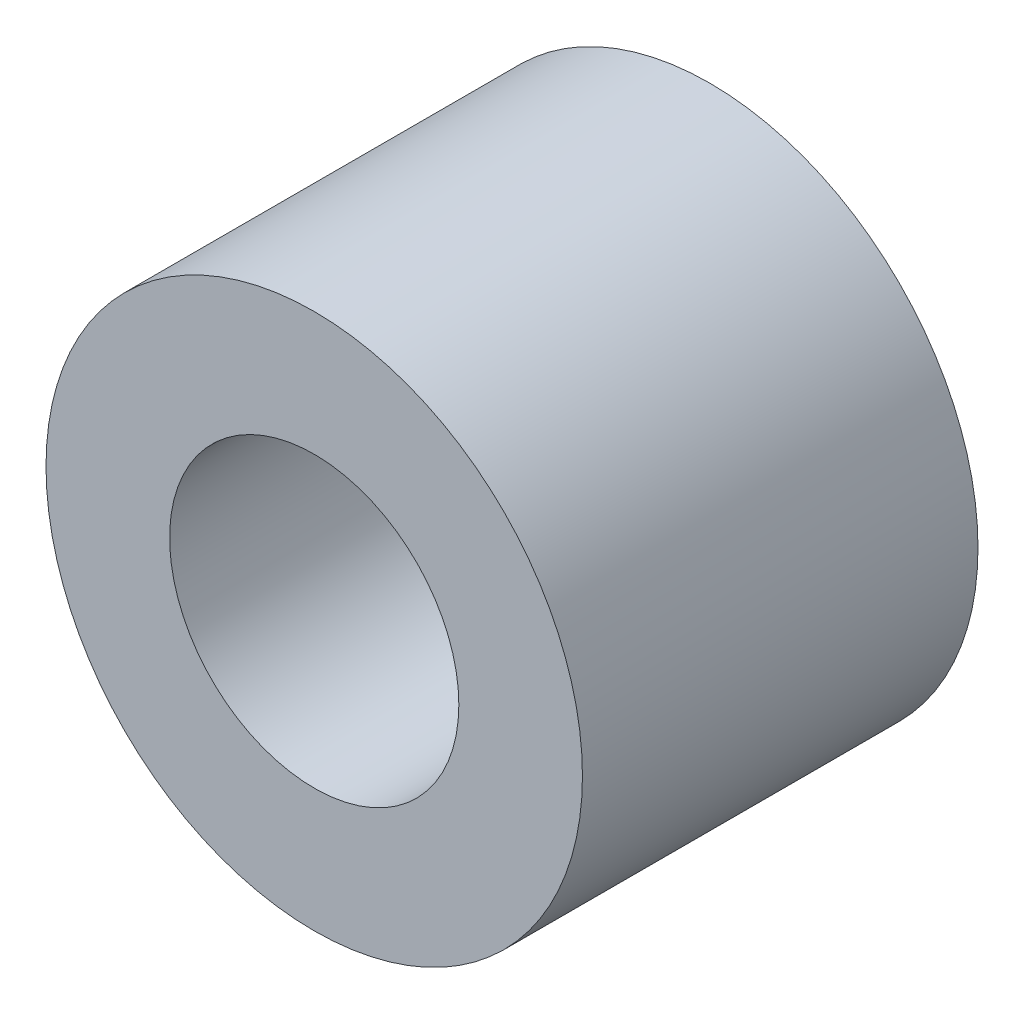
from build123d import *

# Parameters (mm, degrees)
SKETCH1_R           = 10.85
SKETCH1_R_2         = 5.85
BOSS_EXTRUDE1_DEPTH = 16


with BuildPart() as part:
    # Sketch1 → Boss-Extrude1 (new body)
    with BuildSketch(Plane.XY):
        Circle(SKETCH1_R)
        Circle(SKETCH1_R_2, mode=Mode.SUBTRACT)
    extrude(amount=BOSS_EXTRUDE1_DEPTH)


solid = part.part
